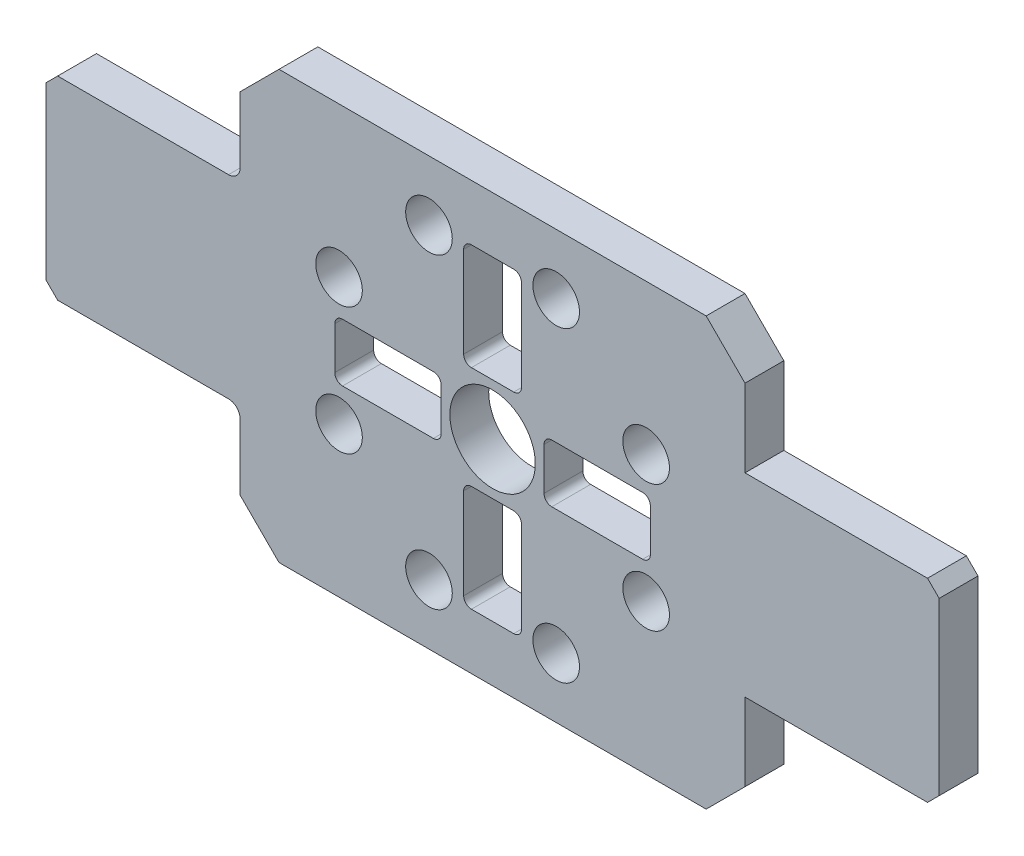
SolidWorks part; units mm, degrees
ref_plane "Front Plane" through (0, 0, 0) normal (0, 0, 1) x (1, 0, 0)
ref_plane "Top Plane" through (0, 0, 0) normal (0, 1, 0) x (1, 0, 0)
ref_plane "Right Plane" through (0, 0, 0) normal (1, 0, 0) x (0, 0, -1)
sketch "Sketch1" plane through (0, 0, 0) normal (0, 0, 1) x (1, 0, 0)
  line L1 (-65, 45) -> (-55, 55)
  line L2 (-55, 55) -> (55, 55)
  line L3 (-65, 45) -> (-65, -45)
  line L4 (-55, -55) -> (55, -55)
  line L5 (65, 45) -> (65, -45)
  line L6 (-65, 55) -> (65, -55) construction
  line L7 (-65, -55) -> (65, 55) construction
  line L8 (-65, -45) -> (-55, -55)
  line L9 (55, -55) -> (65, -45)
  line L10 (55, 55) -> (65, 45)
  line L11 (5.4472, 40.6347) -> (-5.4472, 40.6347)
  line L12 (-7.4472, 38.6347) -> (-7.4472, 15.245)
  line L13 (-5.4472, 13.245) -> (5.4472, 13.245)
  line L14 (7.4472, 15.245) -> (7.4472, 38.6347)
  line L15 (15.245, -7.4472) -> (38.6347, -7.4472)
  line L16 (38.6347, 7.4472) -> (15.245, 7.4472)
  line L17 (40.6347, -5.4472) -> (40.6347, 5.4472)
  line L18 (13.245, 5.4472) -> (13.245, -5.4472)
  line L19 (-7.4472, -15.245) -> (-7.4472, -38.6347)
  line L20 (7.4472, -38.6347) -> (7.4472, -15.245)
  line L21 (-5.4472, -40.6347) -> (5.4472, -40.6347)
  line L22 (5.4472, -13.245) -> (-5.4472, -13.245)
  line L23 (-15.245, 7.4472) -> (-38.6347, 7.4472)
  line L24 (-38.6347, -7.4472) -> (-15.245, -7.4472)
  line L25 (-40.6347, 5.4472) -> (-40.6347, -5.4472)
  line L26 (-13.245, -5.4472) -> (-13.245, 5.4472)
  circle A0 centre (16.3789, 39.542) radius 6
  circle A1 centre (39.542, 16.3789) radius 6
  circle A2 centre (39.542, -16.3789) radius 6
  circle A3 centre (16.3789, -39.542) radius 6
  circle A4 centre (-16.3789, -39.542) radius 6
  circle A5 centre (-39.542, -16.3789) radius 6
  circle A6 centre (-39.542, 16.3789) radius 6
  circle A7 centre (-16.3789, 39.542) radius 6
  arc A8 (5.4472, -40.6347) -> (7.4472, -38.6347) centre (5.4472, -38.6347) ccw
  arc A9 (-5.4472, -40.6347) -> (-7.4472, -38.6347) centre (-5.4472, -38.6347) cw
  arc A10 (-15.245, -7.4472) -> (-13.245, -5.4472) centre (-15.245, -5.4472) ccw
  arc A11 (-38.6347, -7.4472) -> (-40.6347, -5.4472) centre (-38.6347, -5.4472) cw
  arc A12 (-40.6347, 5.4472) -> (-38.6347, 7.4472) centre (-38.6347, 5.4472) cw
  arc A13 (-13.245, 5.4472) -> (-15.245, 7.4472) centre (-15.245, 5.4472) ccw
  arc A14 (-7.4472, -15.245) -> (-5.4472, -13.245) centre (-5.4472, -15.245) cw
  arc A15 (7.4472, -15.245) -> (5.4472, -13.245) centre (5.4472, -15.245) ccw
  arc A16 (40.6347, 5.4472) -> (38.6347, 7.4472) centre (38.6347, 5.4472) ccw
  arc A17 (38.6347, -7.4472) -> (40.6347, -5.4472) centre (38.6347, -5.4472) ccw
  arc A18 (15.245, -7.4472) -> (13.245, -5.4472) centre (15.245, -5.4472) cw
  arc A19 (13.245, 5.4472) -> (15.245, 7.4472) centre (15.245, 5.4472) cw
  arc A20 (5.4472, 13.245) -> (7.4472, 15.245) centre (5.4472, 15.245) ccw
  arc A21 (7.4472, 38.6347) -> (5.4472, 40.6347) centre (5.4472, 38.6347) ccw
  arc A22 (-7.4472, 38.6347) -> (-5.4472, 40.6347) centre (-5.4472, 38.6347) cw
  arc A23 (-7.4472, 15.245) -> (-5.4472, 13.245) centre (-5.4472, 15.245) ccw
  point P0 (0, 0)
  point P33 (0, 0)
  point P52 (0, 0)
  dimension "D3" = 12
  dimension "D10" = 2
  dimension "D1" = 110
  dimension "D2" = 130
  dimension "D9" = 4
  dimension "D4" = 8
extrude "Boss-Extrude1" add sketch "Sketch1" along normal blind 10
sketch "Sketch2" plane through (0, 0, 0) normal (0, 0, 1) x (1, 0, 0)
  line L0 (-65, 45) -> (-65, -45) construction
  line L1 (-112, 25) -> (-65, 25)
  line L2 (-115, 22) -> (-115, -22)
  line L3 (-112, -25) -> (-65, -25)
  line L4 (-65, 25) -> (-65, -25)
  line L5 (-115, 25) -> (-65, -25) construction
  line L6 (-115, -25) -> (-65, 25) construction
  line L7 (90, 0) -> (-90, 0) construction
  line L8 (-115, 22) -> (-112, 25)
  line L9 (-115, -22) -> (-112, -25)
  line L10 (0, 0) -> (0, 112.4317) construction
  line L11 (115, -25) -> (65, 25) construction
  line L12 (115, 25) -> (65, -25) construction
  line L13 (115, -22) -> (112, -25)
  line L14 (115, 22) -> (112, 25)
  line L15 (65, 25) -> (65, -25)
  line L16 (112, -25) -> (65, -25)
  line L17 (115, 22) -> (115, -22)
  line L18 (112, 25) -> (65, 25)
  point P0 (-90, 0)
  point P24 (90, 0)
  dimension "D1" = 50
  dimension "D2" = 50
extrude "Boss-Extrude2" add sketch "Sketch2" along normal up to surface (10 mm away) up to face at (26.9399, 0, 10)
fillet "Fillet1" radius 3 2 edges at (-65, -25, 5) (-65, 25, 5)
sketch "Sketch3" plane through (0, 0, 10) normal (0, 0, 1) x (1, 0, 0)
  circle A0 centre (0, 0) radius 11
  dimension "D1" = 22
extrude "Cut-Extrude1" cut sketch "Sketch3" against normal up to surface (10 mm away) and the other way through all up to face at (-33.542, 16.3789, 0)
